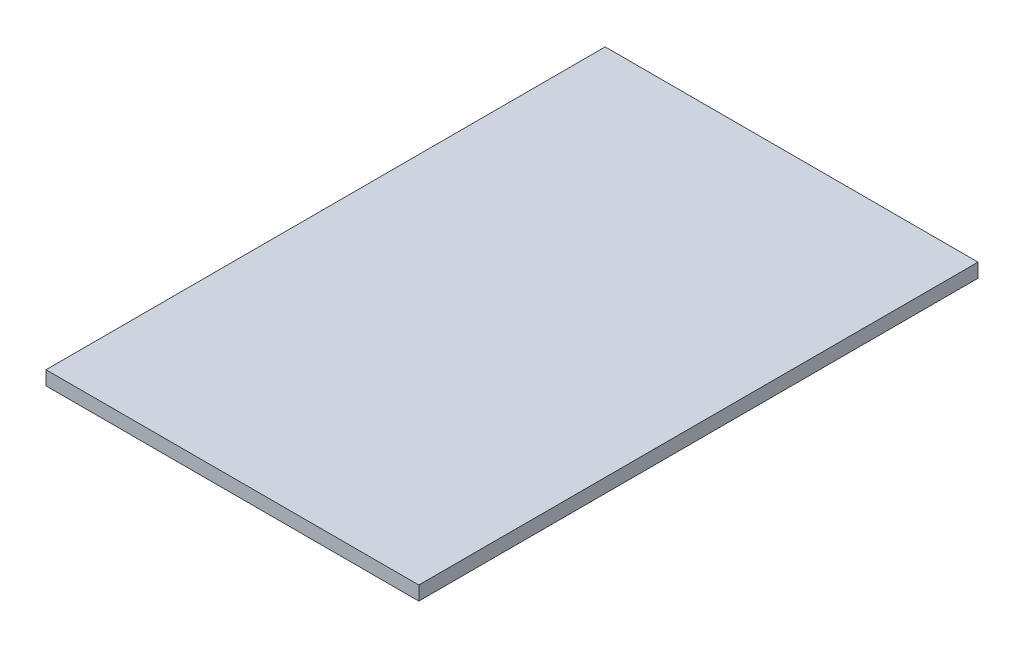
SolidWorks part; units mm, degrees
ref_plane "前视基准面" through (0, 0, 0) normal (0, 0, 1) x (1, 0, 0)
ref_plane "上视基准面" through (0, 0, 0) normal (0, 1, 0) x (1, 0, 0)
ref_plane "右视基准面" through (0, 0, 0) normal (1, 0, 0) x (0, 0, -1)
sketch "草图1" plane through (0, 0, 0) normal (0, 1, 0) x (1, 0, 0)
  line L1 (-400, -600) -> (400, -600)
  line L2 (-400, -600) -> (-400, 600)
  line L3 (-400, 600) -> (400, 600)
  line L4 (400, -600) -> (400, 600)
  line L5 (-400, -600) -> (400, 600) construction
  line L6 (-400, 600) -> (400, -600) construction
  point P0 (0, 0)
  dimension "D1" = 1200
  dimension "D2" = 800
extrude "凸台-拉伸1" add sketch "草图1" along normal blind 30
